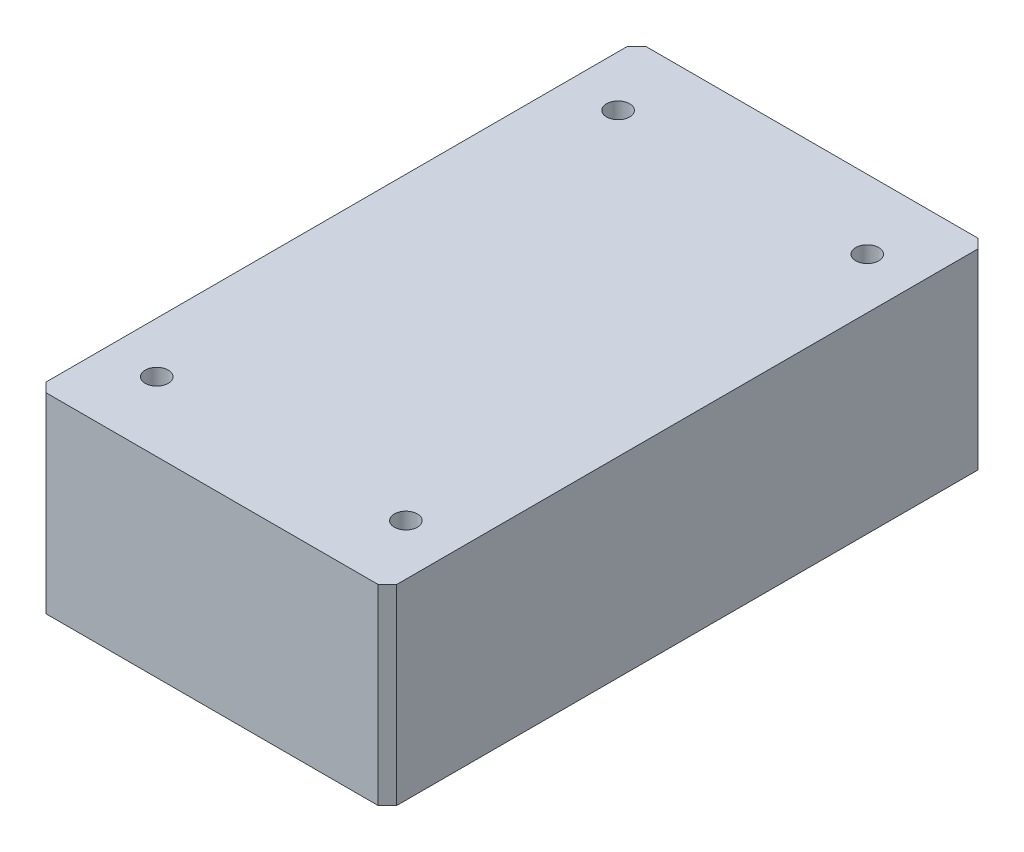
SolidWorks part; units mm, degrees
material "A6061"
ref_plane "前视基准面" through (0, 0, 0) normal (0, 0, 1) x (1, 0, 0)
ref_plane "上视基准面" through (0, 0, 0) normal (0, 1, 0) x (1, 0, 0)
ref_plane "右视基准面" through (0, 0, 0) normal (1, 0, 0) x (0, 0, -1)
sketch "草图1" plane through (0, 0, 0) normal (0, 0, 1) x (1, 0, 0)
  line L1 (-38, 20.75) -> (38, 20.75)
  line L2 (-38, 20.75) -> (-38, -20.75)
  line L3 (-38, -20.75) -> (38, -20.75)
  line L4 (38, 20.75) -> (38, -20.75)
  line L5 (-38, 20.75) -> (38, -20.75) construction
  line L6 (-38, -20.75) -> (38, 20.75) construction
  point P0 (0, 0)
  dimension "D1" = 41.5
  dimension "D2" = 76
extrude "凸台-拉伸1" add sketch "草图1" along normal mid plane 130
hole_wizard "M6 螺纹孔1" positions "草图2" profile "草图3" tap size "M6" standard "GB" end condition through all
sketch "草图2" plane through (0, 20.75, 0) normal (0, 1, 0) x (1, 0, 0)
  line L0 (0, -122.9028) -> (0, 0) construction
  line L1 (0, 0) -> (-70.2302, 0) construction
  point P0 (-27, -50)
  point P9 (27, -50)
  point P10 (27, 50)
  point P11 (-27, 50)
  dimension "D1" = 54
  dimension "D2" = 100
cosmetic thread "孔螺蚊线2"
cosmetic thread "孔螺蚊线3"
cosmetic thread "孔螺蚊线4"
cosmetic thread "孔螺蚊线5"
sketch "草图3" plane through (-27, 20.75, 50) normal (1, 0, 0) x (0, 0, 1)
  line L0 (0, 0) -> (0, 41.5)
  line L1 (0, 41.5) -> (2.5, 41.5)
  line L2 (2.5, 41.5) -> (2.5, 0)
  line L5 (2.5, 0) -> (0, 0)
  line L11 (0, -6.35) -> (0, 107.95) construction
  dimension "通孔螺纹孔钻头直径" = 5
  dimension "通孔螺纹孔钻头深度" = 41.5
chamfer "倒角1" distance 2 angle 45 4 edges at (-38, 0, 65) (38, 0, 65) (-38, 0, -65) (38, 0, -65)
